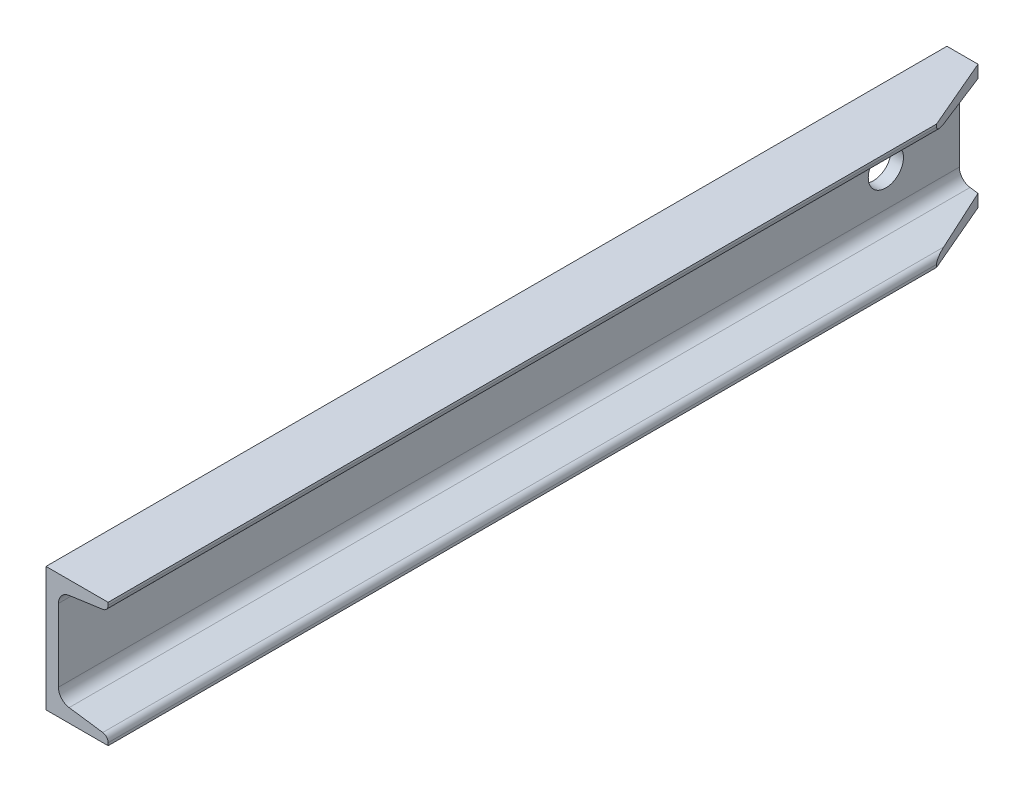
SolidWorks part; units mm, degrees
material "1023 Carbon Steel Plate (SS)"
ref_plane "Front Plane" through (0, 0, 0) normal (0, 0, 1) x (1, 0, 0)
ref_plane "Top Plane" through (0, 0, 0) normal (0, 1, 0) x (1, 0, 0)
ref_plane "Right Plane" through (0, 0, 0) normal (1, 0, 0) x (0, 0, -1)
sketch "Sketch1" plane through (0, 0, 0) normal (0, 0, 1) x (1, 0, 0)
  line L0 (0, 0) -> (-30, 0)
  line L1 (-30, 0) -> (-30, -60)
  line L2 (-30, -60) -> (0, -60)
  line L3 (0, -60) -> (0, -58.716)
  line L4 (-2.5825, -55.7452) -> (-18.835, -53.461)
  line L5 (-24, -47.5194) -> (-24, -12.4806)
  line L6 (-18.835, -6.539) -> (-2.5825, -4.2548)
  line L7 (0, -1.284) -> (0, 0)
  line L8 (-15, -54) -> (-15, -60) construction
  arc A0 (-24, -12.4806) -> (-18.835, -6.539) centre (-18, -12.4806) cw
  arc A1 (-18.835, -53.461) -> (-24, -47.5194) centre (-18, -47.5194) cw
  arc A2 (0, -58.716) -> (-2.5825, -55.7452) centre (-3, -58.716) ccw
  arc A3 (0, -1.284) -> (-2.5825, -4.2548) centre (-3, -1.284) cw
  dimension "D7" = 6
  dimension "D8" = 3
  dimension "D1" = 60
  dimension "D2" = 30
  dimension "D3" = 6
  dimension "D4" = 15
  dimension "D5" = 6
  dimension "D6" = 8
extrude "Boss-Extrude1" add sketch "Sketch1" along normal blind 435 contours A3 L6 A0 L5 A1 L4 A2 L3 L2 L1 L0 L7
sketch "Sketch2" plane through (-30, 0, 0) normal (-1, 0, 0) x (0, 0, 1)
  line L0 (435, 0) -> (435, -60) construction
  circle A0 centre (35.5, -30) radius 8.5
  dimension "D1" = 399.5
  dimension "D2" = 17
extrude "Cut-Extrude1" cut sketch "Sketch2" against normal blind 435
sketch "Sketch3" plane through (0, 0, 0) normal (0, 1, 0) x (1, 0, 0)
  line L0 (-15, 0) -> (0, 0)
  line L2 (0, 0) -> (0, -35)
  line L3 (0, -435) -> (0, 0) construction
  line L4 (0, -35) -> (-15, 0)
  dimension "D1" = 35
  dimension "D2" = 15
extrude "Cut-Extrude2" cut sketch "Sketch3" against normal blind 435
